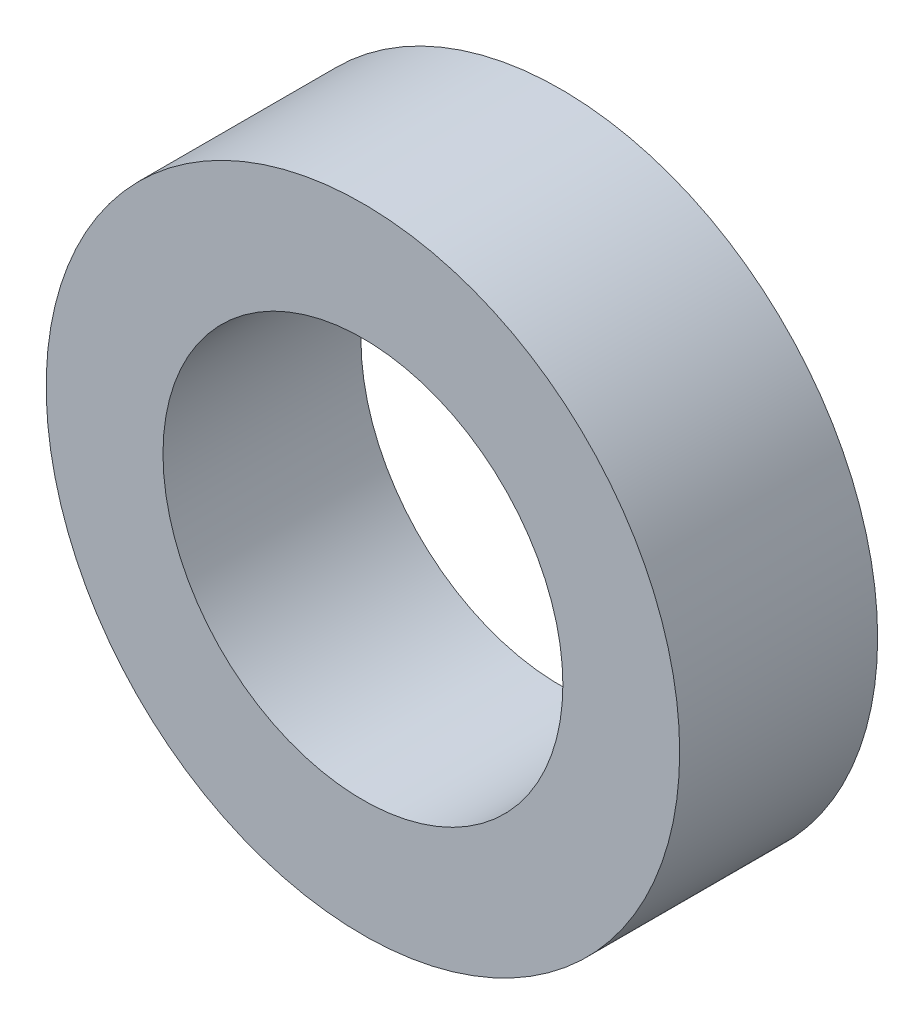
SolidWorks part; units mm, degrees
ref_plane "前视基准面" through (0, 0, 0) normal (0, 0, 1) x (1, 0, 0)
ref_plane "上视基准面" through (0, 0, 0) normal (0, 1, 0) x (1, 0, 0)
ref_plane "右视基准面" through (0, 0, 0) normal (1, 0, 0) x (0, 0, -1)
other "Configuration Table"
sketch "草图1" plane through (0, 0, 0) normal (0, 0, 1) x (1, 0, 0)
  circle A0 centre (0, 0) radius 16
  circle A1 centre (0, 0) radius 10.1
  point P0 (0, 0)
  dimension "D1" = 20.2
  dimension "D2" = 32
extrude "凸台-拉伸1" add sketch "草图1" against normal mid plane 10
